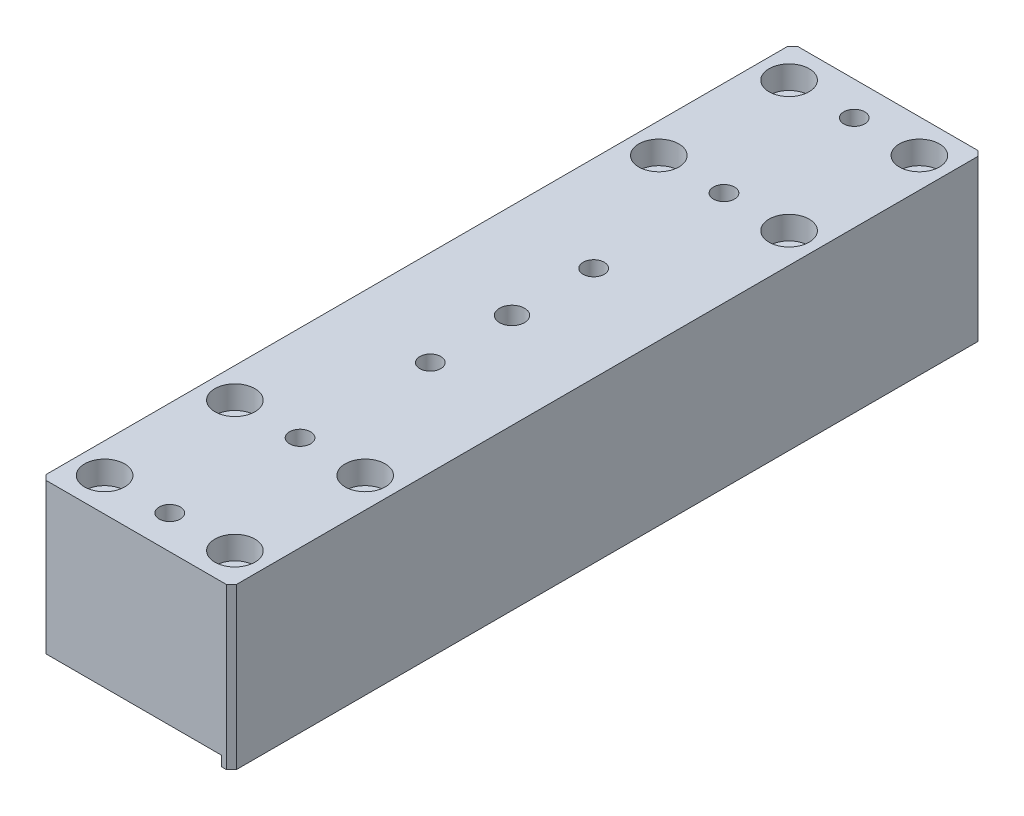
from build123d import *

# Parameters (mm, degrees)
BOSS_EXTRUDE1_DEPTH                                 = 75
HOLE_SIZE_BY_SOCKET_HEAD_CAP_SCREW_TYPE_D           = 4.5
HOLE_SIZE_BY_SOCKET_HEAD_CAP_SCREW_TYPE_CBORE_D     = 8
HOLE_SIZE_BY_SOCKET_HEAD_CAP_SCREW_TYPE_CBORE_DEPTH = 4.6
M5_TAPPED_HOLE1_D                                   = 4.2
M5_TAPPED_HOLE1_DEPTH                               = 12.4
M5_TAPPED_HOLE1_TIP                                 = 1.2618073
M5_TAPPED_HOLE2_D                                   = 4.2
M5_TAPPED_HOLE2_DEPTH                               = 12.4
M5_TAPPED_HOLE2_TIP                                 = 1.2618073
CHAMFER1_SIZE                                       = 1
SIZE_MM_BLIND_PIN_HOLE1_D                           = 5
SIZE_MM_BLIND_PIN_HOLE1_DEPTH                       = 7.5
SIZE_MM_BLIND_PIN_HOLE1_TIP                         = 1.502151548


with BuildPart() as part:
    # Sketch1 → Boss-Extrude1 (new, symmetric)
    with BuildSketch(Plane.XY):
        Polygon((0, 0), (0, 32), (-38, 32), (-38, 2), (-2, 2), (-2, 0), align=None)
    extrude(amount=BOSS_EXTRUDE1_DEPTH, both=True)

    # Hole Size (by socket head cap screw type)1 (through all)
    with Locations(Plane(origin=(0, 32, 0), x_dir=(1, 0, 0), z_dir=(0, 1, 0))):
        with Locations((-32, -68.3), (-32, 68.3), (-6, 42.3), (-32, 42.3), (-6, 68.3), (-6, -68.3), (-6, -42.3), (-32, -42.3)):
            CounterBoreHole(HOLE_SIZE_BY_SOCKET_HEAD_CAP_SCREW_TYPE_D / 2, HOLE_SIZE_BY_SOCKET_HEAD_CAP_SCREW_TYPE_CBORE_D / 2, HOLE_SIZE_BY_SOCKET_HEAD_CAP_SCREW_TYPE_CBORE_DEPTH)

    # M5 Tapped Hole1
    with Locations(Plane(origin=(-38, 0, 0), x_dir=(0, 0, -1), z_dir=(-1, 0, 0))):
        with Locations((0, -17), (-20, -17), (20, -17)):
            Hole(M5_TAPPED_HOLE1_D / 2, depth=M5_TAPPED_HOLE1_DEPTH)
            with Locations((0, 0, -(M5_TAPPED_HOLE1_DEPTH + M5_TAPPED_HOLE1_TIP / 2))):  # 118° drill point
                Cone(0, M5_TAPPED_HOLE1_D / 2, M5_TAPPED_HOLE1_TIP, mode=Mode.SUBTRACT)

    # M5 Tapped Hole2
    with Locations(Plane(origin=(0, 32, 0), x_dir=(1, 0, 0), z_dir=(0, 1, 0))):
        with Locations((-19, -16.3), (-19, 68.3), (-19, 42.3), (-19, -42.3), (-19, -68.3), (-19, 16.3)):
            Hole(M5_TAPPED_HOLE2_D / 2, depth=M5_TAPPED_HOLE2_DEPTH)
            with Locations((0, 0, -(M5_TAPPED_HOLE2_DEPTH + M5_TAPPED_HOLE2_TIP / 2))):  # 118° drill point
                Cone(0, M5_TAPPED_HOLE2_D / 2, M5_TAPPED_HOLE2_TIP, mode=Mode.SUBTRACT)

    # Chamfer1
    chamfer1_edges = [part.edges().sort_by_distance(p)[0] for p in [
        (-38, 17, 75),
        (-38, 17, -75),
        (0, 16, -75),
        (0, 16, 75),
    ]]
    chamfer(chamfer1_edges, length=CHAMFER1_SIZE)

    # Size mm Blind Pin Hole1
    with Locations(Plane(origin=(0, 32, 0), x_dir=(1, 0, 0), z_dir=(0, 1, 0))):
        with Locations((-19, 0)):
            Hole(SIZE_MM_BLIND_PIN_HOLE1_D / 2, depth=SIZE_MM_BLIND_PIN_HOLE1_DEPTH)
            with Locations((0, 0, -(SIZE_MM_BLIND_PIN_HOLE1_DEPTH + SIZE_MM_BLIND_PIN_HOLE1_TIP / 2))):  # 118° drill point
                Cone(0, SIZE_MM_BLIND_PIN_HOLE1_D / 2, SIZE_MM_BLIND_PIN_HOLE1_TIP, mode=Mode.SUBTRACT)


solid = part.part
